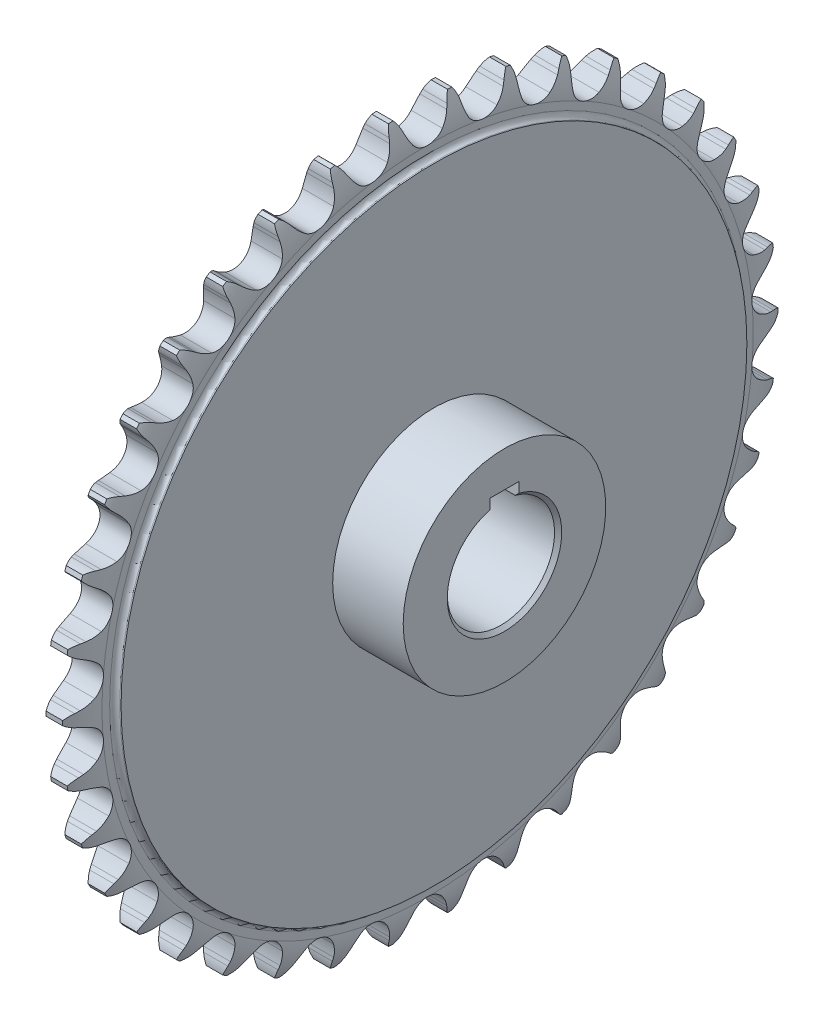
SolidWorks part; units mm, degrees
ref_plane "前视基准面" through (0, 0, 0) normal (0, 0, 1) x (1, 0, 0)
ref_plane "上视基准面" through (0, 0, 0) normal (0, 1, 0) x (1, 0, 0)
ref_plane "右视基准面" through (0, 0, 0) normal (1, 0, 0) x (0, 0, -1)
sketch "草图1" plane through (0, 0, 0) normal (0, 0, 1) x (1, 0, 0)
  line L0 (-7.9375, 0) -> (7.9375, 0) construction
  line L1 (-6.1408, 15) -> (-6.1408, 87.5)
  line L2 (-6.1408, 87.5) -> (-5.7869, 87.5)
  line L3 (-4.371, 88.9159) -> (-4.371, 91.0397)
  line L4 (-2.3072, 100) -> (2.3072, 100)
  line L5 (4.371, 91.0397) -> (4.371, 88.9159)
  line L6 (5.7869, 87.5) -> (6.1408, 87.5)
  line L7 (6.1408, 87.5) -> (6.1408, 15)
  line L8 (6.1408, 15) -> (-6.1408, 15)
  line L9 (0, 0) -> (0, 100) construction
  line L10 (-3.8922, 96.1197) -> (3.8922, 96.1197) construction
  line L11 (-3.8922, -96.1197) -> (3.8922, -96.1197) construction
  line L12 (7.9375, 0) -> (45.9375, 0) construction
  line L13 (-4.371, 91.0397) -> (3.7984, 91.0397) construction
  line L14 (-4.371, -91.0397) -> (3.7984, -91.0397) construction
  line L15 (45.9375, 0) -> (56.0975, 0) construction
  line L16 (56.0975, 0) -> (71.1875, 0) construction
  line L17 (71.1875, 0) -> (80.5875, 0) construction
  line L18 (80.5875, 0) -> (98.6975, 0) construction
  arc A0 (-2.3072, 100) -> (-4.371, 91.0397) centre (11.4679, 92.1095) ccw
  arc A1 (2.3072, 100) -> (4.371, 91.0397) centre (-11.4679, 92.1095) cw
  arc A2 (4.371, 88.9159) -> (5.7869, 87.5) centre (5.7869, 88.9159) ccw
  arc A3 (-5.7869, 87.5) -> (-4.371, 88.9159) centre (-5.7869, 88.9159) ccw
  point P30 (4.371, 87.5)
  point P33 (-4.371, 87.5)
  dimension "D1" = 3.5397
  dimension "rx" = 15.875
  dimension "D3" = 1.4159
  dimension "d" = 192.2394
  dimension "p" = 15.875
  dimension "z" = 38
  dimension "da" = 200
  dimension "df" = 182.0794
  dimension "dr" = 10.16
  dimension "dk" = 30
  dimension "dg" = 175
  dimension "h" = 15.09
  dimension "bf1" = 8.742
  dimension "b1" = 9.4
  dimension "ba" = 2.0638
  dimension "D2" = 1.7698
  dimension "pt" = 18.11
revolve "旋转1" add sketch "草图1" angle 360 about L0
sketch "草图2" plane through (0, 0, 0) normal (1, 0, 0) x (0, 0, -1)
  line L0 (0, 0) -> (0, 100) construction
  line L1 (0, 0) -> (-8.2579, 99.6584) construction
  line L2 (0, 0) -> (-16.4595, 98.6361) construction
  line L3 (4.14, 93.0474) -> (30.5638, 73.4384) construction
  line L4 (5.9511, 96.4087) -> (-6.5271, 100.9634) construction
  line L5 (0, 0) -> (8.2579, 99.6584) construction
  line L6 (5.9511, 96.4087) -> (6.3545, 97.5141)
  line L7 (-5.9511, 96.4087) -> (-6.3545, 97.5141)
  circle A0 centre (0, 0) radius 100 construction
  arc A1 (4.14, 93.0474) -> (-4.14, 93.0474) centre (0, 96.1197) cw
  arc A2 (4.14, 93.0474) -> (5.9511, 96.4087) centre (-6.5271, 100.9634) ccw
  arc A3 (7.6284, 99.7086) -> (6.3545, 97.5141) centre (13.1629, 95.029) ccw
  arc A4 (-4.14, 93.0474) -> (-5.9511, 96.4087) centre (6.5271, 100.9634) cw
  arc A5 (-7.6284, 99.7086) -> (-6.3545, 97.5141) centre (-13.1629, 95.029) cw
  arc A7 (7.6284, 99.7086) -> (-7.6284, 99.7086) centre (0, 0) ccw
  dimension "r1" = 5.1554
  dimension "r3" = 7.2477
  dimension "D1" = 9.474
  dimension "D2" = 4.737
  dimension "α/2" = 53.421
  dimension "M" = 6.5271
  dimension "T" = 4.8437
  dimension "β" = 16.526
  dimension "γ/2" = 15.316
  dimension "bc" = 1.1767
extrude "切除-拉伸1" cut sketch "草图2" against normal mid plane 12.2817
pattern_circular "阵列(圆周)1" count 38 over 360 about axis through (0, 0, 0) along (1, 0, 0) of "切除-拉伸1"
sketch "草图3" plane through (0, 0, 0) normal (0, 0, 1) x (1, 0, 0)
  line L0 (6.1408, 15) -> (25.8592, 15)
  line L3 (25.8592, 15) -> (25.8592, 28.3224)
  line L4 (25.8592, 28.3224) -> (6.1408, 28.3224)
  line L5 (6.1408, 28.3224) -> (6.1408, 15)
  line L6 (0, 0) -> (6.4, 0) construction
  line L8 (-6.1408, 87.5) -> (-6.1408, -87.5) construction
  dimension "h" = 13.3224
  dimension "K" = 6.4
  dimension "L" = 32
revolve "旋转2" add sketch "草图3" angle 360 about L6
sketch "草图4" plane through (-6.1408, 0, 0) normal (-1, 0, 0) x (0, 0, 1)
  line L1 (-4, 14.4568) -> (4, 14.4568)
  line L2 (-4, 14.4568) -> (-4, 18.3)
  line L3 (-4, 18.3) -> (4, 18.3)
  line L4 (4, 14.4568) -> (4, 18.3)
  circle A0 centre (0, 0) radius 15 construction
  point P6 (0.7, 18.3)
  dimension "D1" = 18.3
  dimension "键槽宽度" = 8
  dimension "t1" = 3.3
extrude "切除-拉伸2" cut sketch "草图4" against normal through all
chamfer "倒角1" distance 1 angle 45 1 edges at (-6.1408, -15, 0)
chamfer "倒角3" distance 1 angle 45 1 edges at (25.8592, -15, 0)
